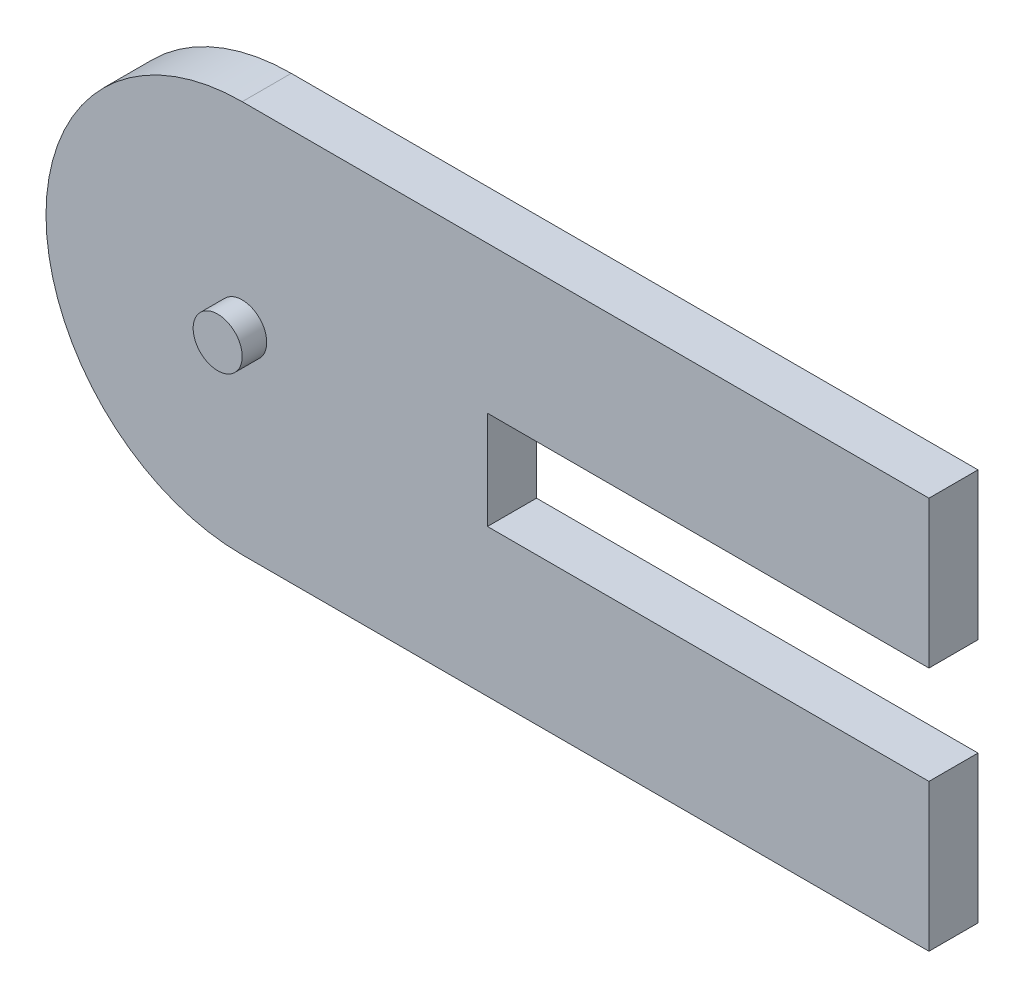
from build123d import *

# Parameters (mm, degrees)
BASE_EXTRUDE_DEPTH  = 10
SKETCH2_R           = 5
BOSS_EXTRUDE1_DEPTH = 5


with BuildPart() as part:
    # Sketch1 → Base-Extrude (new body)
    with BuildSketch(Plane.XY):
        with BuildLine():
            Line((0, 40), (140, 40))
            Line((140, 40), (140, 10))
            Line((140, 10), (50, 10))
            Line((50, 10), (50, -10))
            Line((50, -10), (140, -10))
            Line((140, -10), (140, -40))
            Line((140, -40), (0, -40))
            ThreePointArc((0, -40), (-40, 0), (0, 40))
        make_face()
    extrude(amount=BASE_EXTRUDE_DEPTH)

    # Sketch2 → Boss-Extrude1 (add)
    with BuildSketch(Plane.XY.offset(10)):
        Circle(SKETCH2_R)
    extrude(amount=BOSS_EXTRUDE1_DEPTH)


solid = part.part
